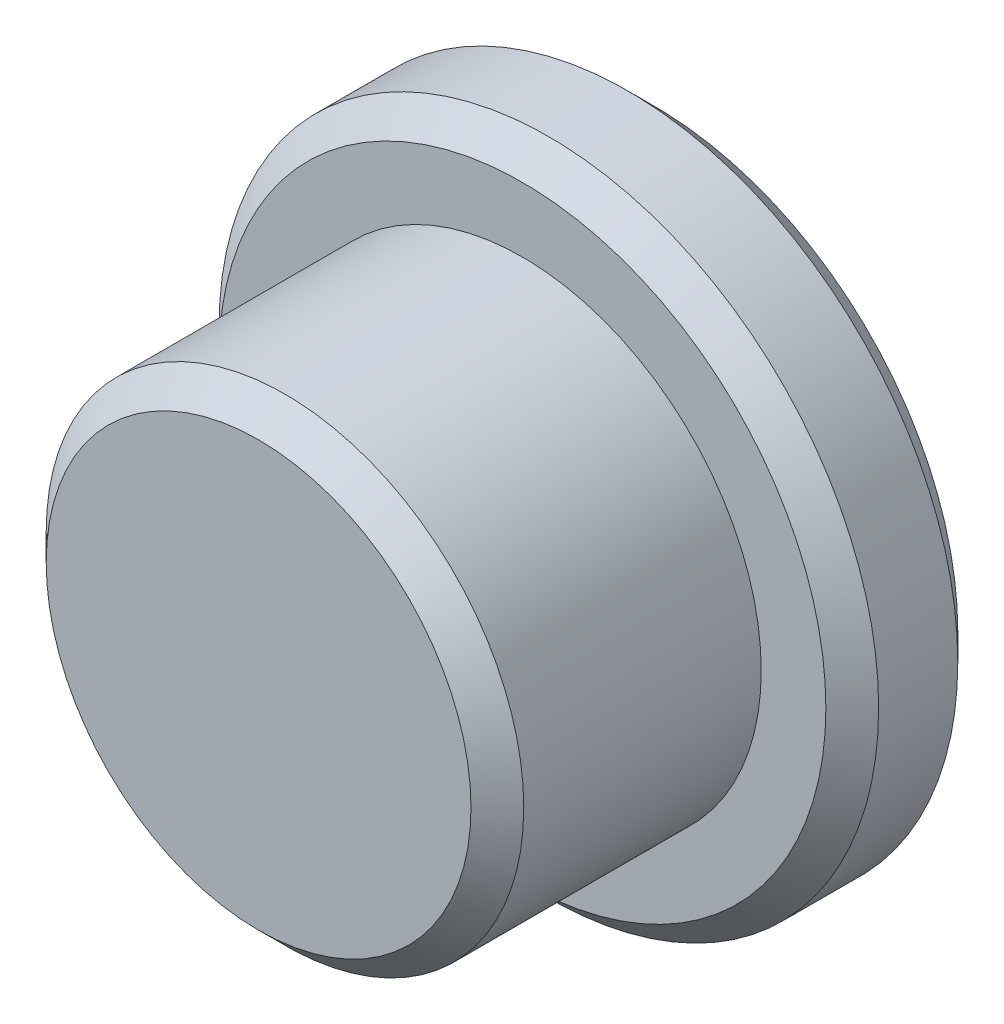
SolidWorks part; units mm, degrees
material "Q235B"
ref_plane "Front Plane" through (0, 0, 0) normal (0, 0, 1) x (1, 0, 0)
ref_plane "Top Plane" through (0, 0, 0) normal (0, 1, 0) x (1, 0, 0)
ref_plane "Right Plane" through (0, 0, 0) normal (1, 0, 0) x (0, 0, -1)
sketch "Sketch1" plane through (0, 0, 0) normal (1, 0, 0) x (0, 0, -1)
  line L0 (0, 0) -> (15, 0) construction
  line L1 (15, 0) -> (15, 12.5)
  line L2 (15, 12.5) -> (10, 12.5)
  line L3 (10, 12.5) -> (10, 9.05)
  line L4 (10, 9.05) -> (0, 9.05)
  line L7 (0, 9.05) -> (0, 0)
  line L8 (0, 0) -> (15, 0)
  dimension "D2" = 18.1
  dimension "D3" = 25
  dimension "D4" = 5
  dimension "D5" = 10
revolve "Revolve1" add sketch "Sketch1" angle 360 about L0
chamfer "Chamfer1" distance 1 angle 45 3 edges at (12.5, 0, -15) (12.5, 0, -10) (9.05, 0, 0)
